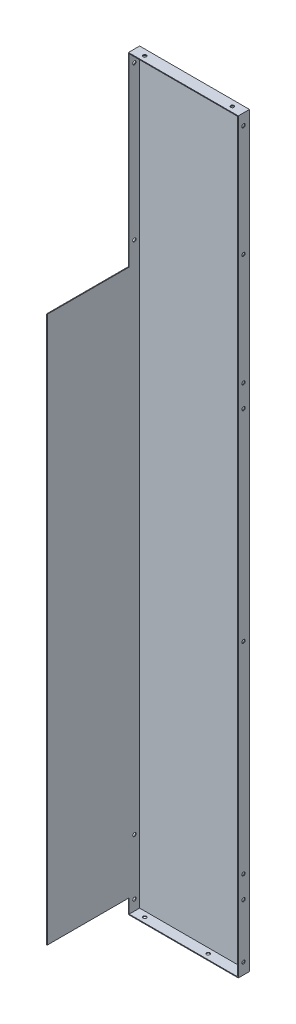
SolidWorks part; units mm, degrees
ref_plane "前视基准面" through (0, 0, 0) normal (0, 0, 1) x (1, 0, 0)
ref_plane "上视基准面" through (0, 0, 0) normal (0, 1, 0) x (1, 0, 0)
ref_plane "右视基准面" through (0, 0, 0) normal (1, 0, 0) x (0, 0, -1)
sketch "草图1" plane through (0, 0, 0) normal (0, 0, 1) x (1, 0, 0)
  line L1 (0, 0) -> (295, 0)
  line L2 (0, 0) -> (0, 2005)
  line L3 (0, 2005) -> (295, 2005)
  line L4 (295, 0) -> (295, 2005)
  dimension "D1" = 295
  dimension "D2" = 2005
extrude "凸台-拉伸1" add sketch "草图1" along normal blind 30
shell "抽壳1" thickness 2
sketch "草图2" plane through (0, 0, 30) normal (0, 0, 1) x (1, 0, 0)
  line L0 (0, 2005) -> (0, 0) construction
  line L1 (0, 1507) -> (2, 1507)
  line L2 (0, 1507) -> (0, 40)
  line L3 (0, 40) -> (2, 40)
  line L4 (2, 1507) -> (2, 40)
  line L5 (2, 2003) -> (2, 2) construction
  line L6 (0, 0) -> (295, 0) construction
  dimension "D1" = 40
  dimension "D2" = 1467
extrude "凸台-拉伸2" add sketch "草图2" along normal blind 220
sketch "草图3" plane through (0, 2, 0) normal (0, 1, 0) x (1, 0, 0)
  line L0 (2, -16) -> (332.0381, -16) construction
  line L1 (2, -30) -> (2, -2) construction
  line L2 (0, -30) -> (0, 0) construction
  circle A0 centre (30, -16) radius 4.5
  circle A1 centre (200, -16) radius 4.5
  dimension "D1" = 9
  dimension "D2" = 9
  dimension "D3" = 30
  dimension "D4" = 170
extrude "切除-拉伸1" cut sketch "草图3" against normal blind 10
sketch "草图4" plane through (2, 0, 0) normal (1, 0, 0) x (0, 0, -1)
  line L0 (-16, 2) -> (-16, 192.3894) construction
  line L1 (-30, 2) -> (-2, 2) construction
  line L2 (-30, 0) -> (0, 0) construction
  circle A0 centre (-16, 30) radius 4.5
  circle A1 centre (-16, 180) radius 4.5
  dimension "D1" = 9
  dimension "D2" = 9
  dimension "D3" = 150
  dimension "D4" = 30
extrude "切除-拉伸2" cut sketch "草图4" against normal blind 116
sketch "草图5" plane through (2, 0, 0) normal (1, 0, 0) x (0, 0, -1)
  line L0 (-16, 2003) -> (-16, 1559.5737) construction
  line L1 (-30, 2003) -> (-2, 2003) construction
  line L2 (-30, 2005) -> (0, 2005) construction
  circle A0 centre (-16, 1975) radius 4.5
  circle A1 centre (-16, 1563) radius 4.5
  dimension "D1" = 9
  dimension "D2" = 9
  dimension "D3" = 412
  dimension "D4" = 30
extrude "切除-拉伸3" cut sketch "草图5" against normal blind 72
sketch "草图6" plane through (0, 2005, 0) normal (0, 1, 0) x (1, 0, 0)
  line L1 (295, -30) -> (295, 0) construction
  line L2 (295, -16) -> (0, -16)
  line L3 (295, -16) -> (0, -16) construction
  line L4 (0, -30) -> (0, 0) construction
  circle A0 centre (30, -16) radius 4.5
  circle A1 centre (265, -16) radius 4.5
  dimension "D2" = 9
  dimension "D3" = 9
  dimension "D4" = 30
  dimension "D5" = 30
  dimension "D1" = 14
extrude "切除-拉伸4" cut sketch "草图6" against normal blind 10
sketch "草图7" plane through (293, 0, 0) normal (-1, 0, 0) x (0, 0, 1)
  line L0 (16, 2003) -> (16, 10.1346) construction
  line L1 (30, 2003) -> (2, 2003) construction
  line L2 (30, 2005) -> (0, 2005) construction
  circle A0 centre (16, 1975) radius 4.5
  circle A1 centre (16, 1676) radius 4.5
  circle A2 centre (16, 1377) radius 4.5
  circle A3 centre (16, 1317) radius 4.5
  circle A4 centre (16, 776) radius 4.5
  circle A5 centre (16, 235) radius 4.5
  dimension "D1" = 9
  dimension "D2" = 9
  dimension "D3" = 9
  dimension "D4" = 30
  dimension "D5" = 598
  dimension "D6" = 299
  dimension "D7" = 9
  dimension "D8" = 9
  dimension "D9" = 9
  dimension "D10" = 60
  dimension "D11" = 1082
  dimension "D12" = 541
extrude "切除-拉伸5" cut sketch "草图7" against normal blind 10
sketch "草图8" plane through (295, 0, 0) normal (1, 0, 0) x (0, 0, -1)
  line L1 (-30, 0) -> (0, 0) construction
  line L2 (-16, 0) -> (-16, 2005)
  line L3 (-16, 0) -> (-16, 2005) construction
  circle A0 centre (-16, 30) radius 4.5
  circle A1 centre (-16, 175) radius 4.5
  dimension "D2" = 9
  dimension "D3" = 9
  dimension "D4" = 30
  dimension "D5" = 145
  dimension "D1" = 14
extrude "切除-拉伸6" cut sketch "草图8" against normal blind 16
